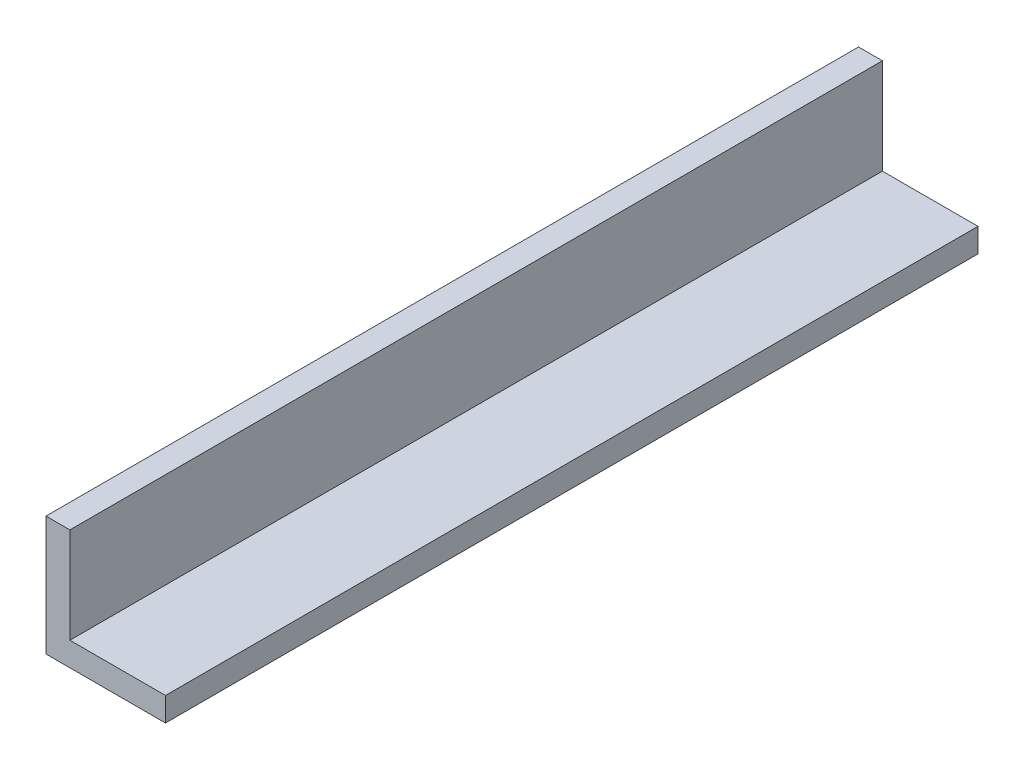
from build123d import *

# Parameters (mm, degrees)
EXTRUDE_1_DEPTH = 170


with BuildPart() as part:
    # 草图1 → 凸台-拉伸1 (new body)
    with BuildSketch(Plane.XY):
        Polygon((0, 0), (0, 25), (5, 25), (5, 5), (25, 5), (25, 0), align=None)
    extrude(amount=EXTRUDE_1_DEPTH)


solid = part.part
